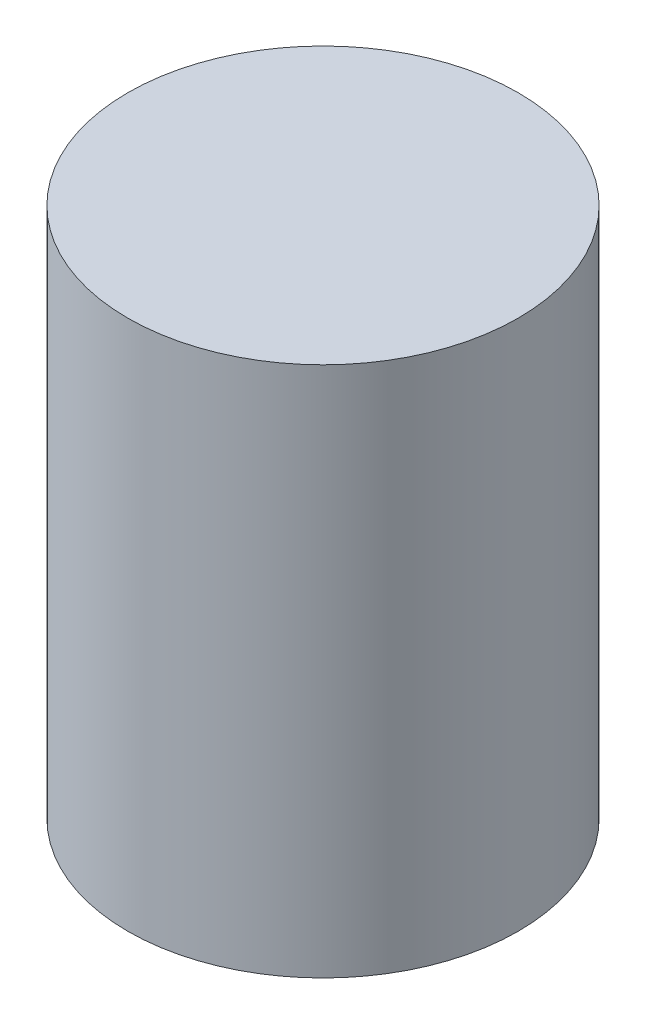
from build123d import *

# Parameters (mm, degrees)
SKETCH_1_R      = 12.5
EXTRUDE_1_DEPTH = 34


with BuildPart() as part:
    # 草图1 → 凸台-拉伸1 (new body)
    with BuildSketch(Plane(origin=(0, 0, 0), x_dir=(1, 0, 0), z_dir=(0, 1, 0))):
        with Locations(Location((0, 0, 0), (0, 0, 270))):
            Circle(SKETCH_1_R)
    extrude(amount=EXTRUDE_1_DEPTH)


solid = part.part
